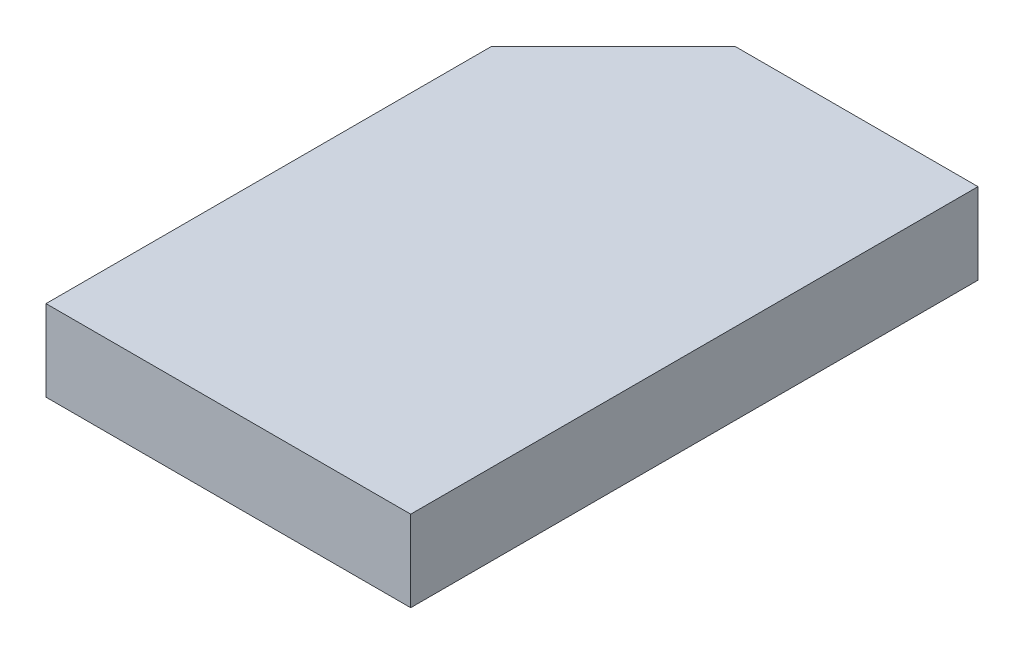
SolidWorks part; units mm, degrees
ref_plane "Front Plane" through (0, 0, 0) normal (0, 0, 1) x (1, 0, 0)
ref_plane "Top Plane" through (0, 0, 0) normal (0, 1, 0) x (1, 0, 0)
ref_plane "Right Plane" through (0, 0, 0) normal (1, 0, 0) x (0, 0, -1)
sketch "Sketch1" plane through (0, 0, 0) normal (0, 1, 0) x (1, 0, 0)
  line L0 (-90, 110) -> (-60, 140)
  line L1 (0, 0) -> (-90, 0)
  line L2 (0, 0) -> (0, 140)
  line L3 (0, 140) -> (-60, 140)
  line L4 (-90, 0) -> (-90, 110)
  dimension "D1" = 110
  dimension "D2" = 140
  dimension "D3" = 90
  dimension "D4" = 60
extrude "Boss-Extrude1" add sketch "Sketch1" along normal blind 20
